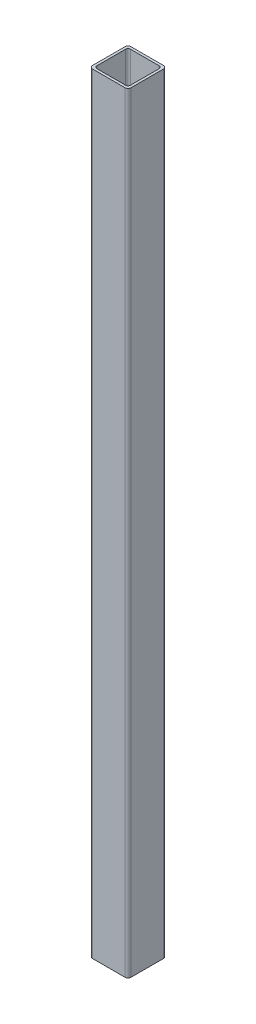
SolidWorks part; units mm, degrees
material "Angle steel 100×100×6/Q235"
ref_plane "Front Plane" through (0, 0, 0) normal (0, 0, 1) x (1, 0, 0)
ref_plane "Top Plane" through (0, 0, 0) normal (0, 1, 0) x (1, 0, 0)
ref_plane "Right Plane" through (0, 0, 0) normal (1, 0, 0) x (0, 0, -1)
sketch "Sketch2" plane through (0, 0, 0) normal (0, 1, 0) x (1, 0, 0)
  line L0 (12.6, 4.775) -> (87.4, 4.775)
  line L1 (6.3, 11.075) -> (6.3, 85.875)
  line L2 (87.4, 92.175) -> (12.6, 92.175)
  line L3 (93.7, 85.875) -> (93.7, 11.075)
  line L4 (7.875, -1.525) -> (92.125, -1.525)
  line L5 (0, 6.35) -> (0, 90.6)
  line L6 (92.125, 98.475) -> (7.875, 98.475)
  line L7 (100, 90.6) -> (100, 6.35)
  arc A0 (100, 90.6) -> (92.125, 98.475) centre (92.125, 90.6) ccw
  arc A1 (92.125, -1.525) -> (100, 6.35) centre (92.125, 6.35) ccw
  arc A2 (0, 6.35) -> (7.875, -1.525) centre (7.875, 6.35) ccw
  arc A3 (7.875, 98.475) -> (0, 90.6) centre (7.875, 90.6) ccw
  arc A4 (12.6, 92.175) -> (6.3, 85.875) centre (12.6, 85.875) ccw
  arc A5 (93.7, 85.875) -> (87.4, 92.175) centre (87.4, 85.875) ccw
  arc A6 (87.4, 4.775) -> (93.7, 11.075) centre (87.4, 11.075) ccw
  arc A7 (6.3, 11.075) -> (12.6, 4.775) centre (12.6, 11.075) ccw
extrude "Boss-Extrude1" add sketch "Sketch2" along normal mid plane 2000
